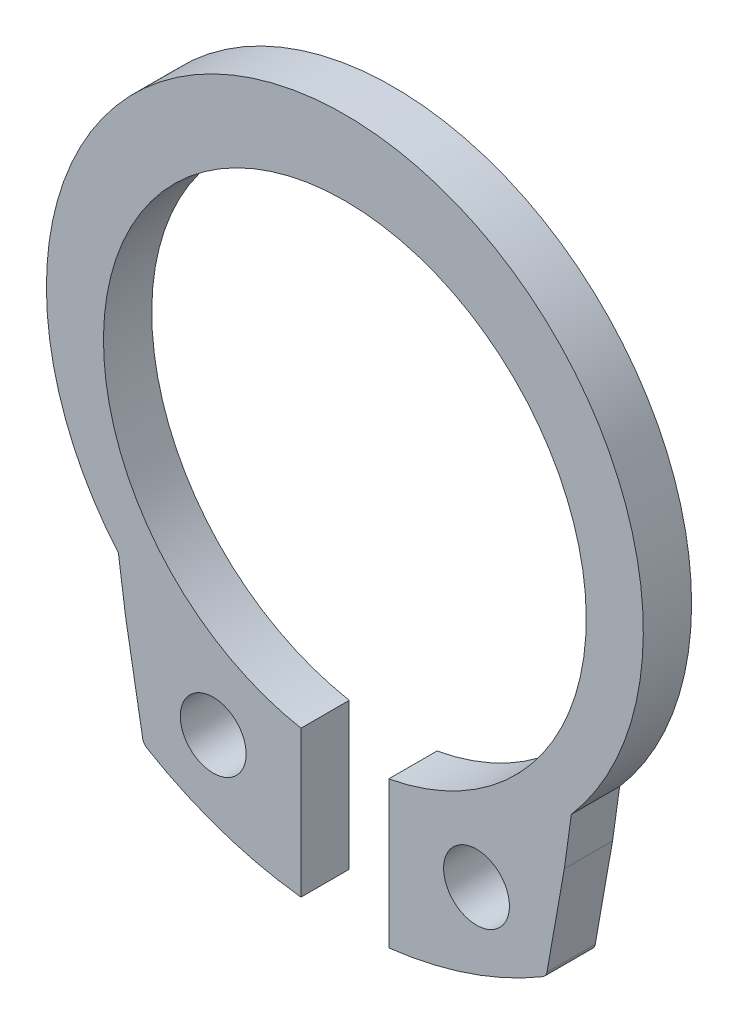
SolidWorks part; units mm, degrees
ref_plane "Front Plane" through (0, 0, 0) normal (0, 0, 1) x (1, 0, 0)
ref_plane "Top Plane" through (0, 0, 0) normal (0, 1, 0) x (1, 0, 0)
ref_plane "Right Plane" through (0, 0, 0) normal (1, 0, 0) x (0, 0, -1)
other "Configuration Table"
sketch "Sketch1" plane through (0, 0, 0) normal (0, 0, 1) x (1, 0, 0)
  line L0 (-13.5503, 0.4) -> (16.7203, 0.4) construction
  line L1 (0, 9.6214) -> (0, -3.5715) construction
  line L3 (1, -6.3261) -> (1, -4.8403)
  line L4 (-5, -5.1807) -> (-4.6053, -7.4189)
  line L5 (-1, -7.1302) -> (-1, -5.4083)
  line L6 (-1, -4.0283) -> (0.0032, -4.0283)
  line L7 (-1, -7.1302) -> (-1, -8.743)
  line L8 (1, -7.1302) -> (1, -8.743)
  line L9 (5, -5.1807) -> (4.6053, -7.4189)
  line L10 (-5, -5.1807) -> (-5.1605, -4.0283)
  line L11 (-0.42, -3.1656) -> (0.0032, -4.0283)
  line L12 (1, -6.3261) -> (1, -7.1302)
  line L13 (5, -5.1807) -> (5.1605, -4.0283)
  arc A1 (5.1605, -4.0283) -> (-5.1605, -4.0283) centre (0, 0.4) ccw
  arc A2 (1, -5.4083) -> (-1, -5.4083) centre (0, 0) ccw
  arc A3 (-4.5109, -7.5559) -> (-1, -8.743) centre (0, 0) ccw
  arc A4 (1, -8.743) -> (4.5109, -7.5559) centre (0, 0) ccw
  arc A7 (4.5109, -7.5559) -> (4.6053, -7.4189) centre (4.4084, -7.3842) ccw
  arc A8 (-4.5109, -7.5559) -> (-4.6053, -7.4189) centre (-4.4084, -7.3842) cw
  circle A9 centre (-3, -6.5452) radius 0.75
  circle A10 centre (3, -6.5452) radius 0.75
  dimension "D4" = 13.6
  dimension "D5" = 11
  dimension "D6" = 17.6
  dimension "D7" = 0.2
  dimension "D8" = 1.5
  dimension "D11" = 1.5
  dimension "D2" = 0.4
  dimension "D3" = 0.4
  dimension "D9" = 2
  dimension "D10" = 1
  dimension "D12" = 6
  dimension "D13" = 3
  dimension "D14" = 0
extrude "Boss-Extrude1" add sketch "Sketch1" along normal blind 1.1 contours A8 A3 L7 L5 A2 L3 L12 L8 A4 A7 L9 L13 A1 L10 L4 A10 A9
